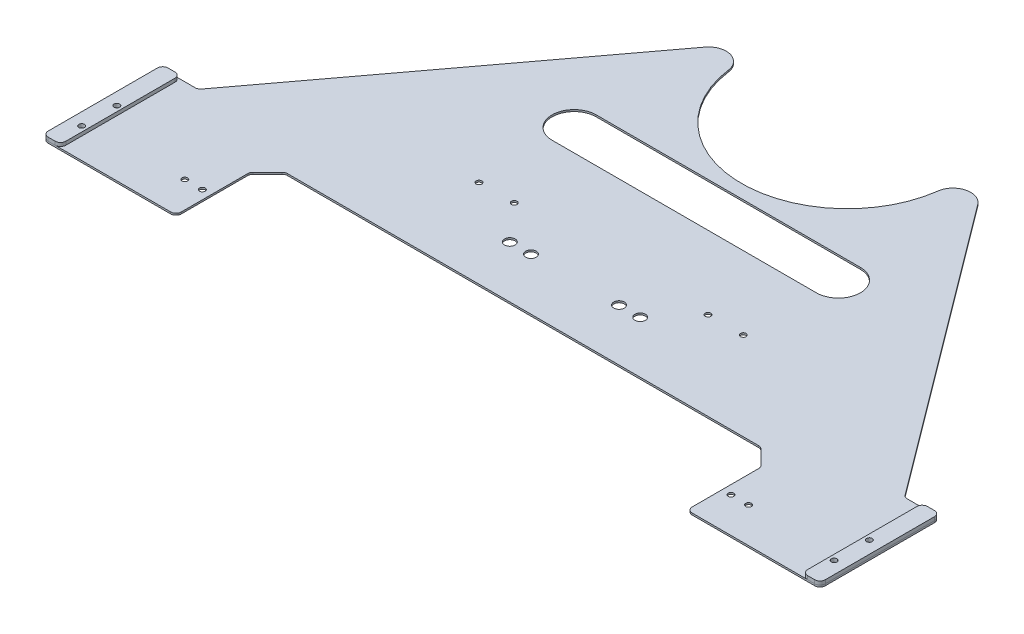
from build123d import *

# Parameters (mm, degrees)
SKETCH_1_R          = 1.6
EXTRUDE_1_DEPTH     = 1
SKETCH_2_R          = 1.6
SKETCH_2_R_2        = 3
CUT_EXTRUDE_1_DEPTH = 10
FILLET_1_R          = 3
SKETCH_3_R          = 1.6
EXTRUDE_2_DEPTH     = 2


with BuildPart() as part:
    # 草图1 → 凸台-拉伸1 (new body)
    with BuildSketch(Plane(origin=(0, 0, 0), x_dir=(1, 0, 0), z_dir=(0, 1, 0))):
        with BuildLine():
            Line((-135, 52), (135, 52))
            Line((135, 52), (145, 42))
            Line((145, 42), (145, 0))
            Line((145, 0), (220.55, 0))
            Line((220.55, 0), (220.55, 68))
            Line((220.55, 68), (200.55, 68))
            Line((200.55, 68), (77.389287954, 232.698771447))
            ThreePointArc((77.389287954, 232.698771447), (66.863287332, 236.388001217), (59.469269979, 228.037216058))
            ThreePointArc((59.469269979, 228.037216058), (0, 176), (-59.469269979, 228.037216058))
            ThreePointArc((-59.469269979, 228.037216058), (-66.863287332, 236.388001217), (-77.389287954, 232.698771447))
            Line((-77.389287954, 232.698771447), (-200.55, 68))
            Line((-200.55, 68), (-220.55, 68))
            Line((-220.55, 68), (-220.55, 0))
            Line((-220.55, 0), (-145, 0))
            Line((-145, 0), (-145, 42))
            Line((-145, 42), (-135, 52))
        make_face()
        with Locations(Location((213.55, 35, 0), (0, 0, 270))):
            Circle(SKETCH_1_R, mode=Mode.SUBTRACT)
        with Locations(Location((-213.55, 35, 0), (0, 0, 90))):
            Circle(SKETCH_1_R, mode=Mode.SUBTRACT)
        with Locations(Location((213.55, 15, 0), (0, 0, 270))):
            Circle(SKETCH_1_R, mode=Mode.SUBTRACT)
        with Locations(Location((-213.55, 15, 0), (0, 0, 90))):
            Circle(SKETCH_1_R, mode=Mode.SUBTRACT)
    extrude(amount=EXTRUDE_1_DEPTH)

    # 草图2 → 切除-拉伸1 (cut)
    with BuildSketch(Plane(origin=(0, 1, 0), x_dir=(1, 0, 0), z_dir=(0, 1, 0))):
        with Locations(Location((-55, 102, 0), (0, 0, 270))):
            Circle(SKETCH_2_R)
        with Locations(Location((-75, 102, 0), (0, 0, 270))):
            Circle(SKETCH_2_R)
        with Locations(Location((75, 102, 0), (0, 0, 270))):
            Circle(SKETCH_2_R)
        with Locations(Location((55, 102, 0), (0, 0, 270))):
            Circle(SKETCH_2_R)
        with Locations(Location((-25, 81.5, 0), (0, 0, 270))):
            Circle(SKETCH_2_R_2)
        with Locations(Location((-37, 81.5, 0), (0, 0, 270))):
            Circle(SKETCH_2_R_2)
        with Locations(Location((37, 81.5, 0), (0, 0, 270))):
            Circle(SKETCH_2_R_2)
        with Locations(Location((25, 81.5, 0), (0, 0, 270))):
            Circle(SKETCH_2_R_2)
        with Locations(Location((-160, 20, 0), (0, 0, 270))):
            Circle(SKETCH_2_R)
        with Locations(Location((-150, 20, 0), (0, 0, 270))):
            Circle(SKETCH_2_R)
        with Locations(Location((150, 20, 0), (0, 0, 270))):
            Circle(SKETCH_2_R)
        with Locations(Location((160, 20, 0), (0, 0, 270))):
            Circle(SKETCH_2_R)
        with BuildLine():
            Line((-75, 168.5), (75, 168.5))
            ThreePointArc((75, 168.5), (87.5, 156), (75, 143.5))
            Line((75, 143.5), (-75, 143.5))
            ThreePointArc((-75, 143.5), (-87.5, 156), (-75, 168.5))
        make_face()
    extrude(amount=-CUT_EXTRUDE_1_DEPTH, mode=Mode.SUBTRACT)

    # 圆角1
    fillet_1_edges = [part.edges().sort_by_distance(p)[0] for p in [
        (145, 0.5, 0),
        (145, 0.5, -42),
        (135, 0.5, -52),
        (-135, 0.5, -52),
        (-145, 0.5, -42),
        (-145, 0.5, 0),
        (-220.55, 0.5, 0),
        (-220.55, 0.5, -68),
        (-200.55, 0.5, -68),
        (200.55, 0.5, -68),
        (220.55, 0.5, -68),
        (220.55, 0.5, 0),
    ]]
    fillet(fillet_1_edges, radius=FILLET_1_R)


with BuildPart() as body_2:
    # 草图3 → 凸台-拉伸2 (new body)
    with BuildSketch(Plane(origin=(0, 1, 0), x_dir=(1, 0, 0), z_dir=(0, 1, 0))):
        with BuildLine():
            Line((213.55, 0), (217.55, 0))
            ThreePointArc((217.55, 0), (219.671320344, 0.878679656), (220.55, 3))
            Line((220.55, 3), (220.55, 65))
            ThreePointArc((220.55, 65), (219.671320344, 67.121320344), (217.55, 68))
            Line((217.55, 68), (213.55, 68))
            ThreePointArc((213.55, 68), (211.428679656, 67.121320344), (210.55, 65))
            Line((210.55, 65), (210.55, 3))
            ThreePointArc((210.55, 3), (211.428679656, 0.878679656), (213.55, 0))
        make_face()
        with Locations(Location((213.55, 15, 0), (0, 0, 270))):
            Circle(SKETCH_3_R, mode=Mode.SUBTRACT)
        with Locations(Location((213.55, 35, 0), (0, 0, 270))):
            Circle(SKETCH_3_R, mode=Mode.SUBTRACT)
    extrude(amount=EXTRUDE_2_DEPTH)


with BuildPart() as body_3:
    # 镜向1: mirrored copy
    add(body_2.part.mirror(Plane(origin=(0, 0, 0), x_dir=(0, 0, 1), z_dir=(1, 0, 0))))


solid = Compound([part.part, body_2.part, body_3.part])
